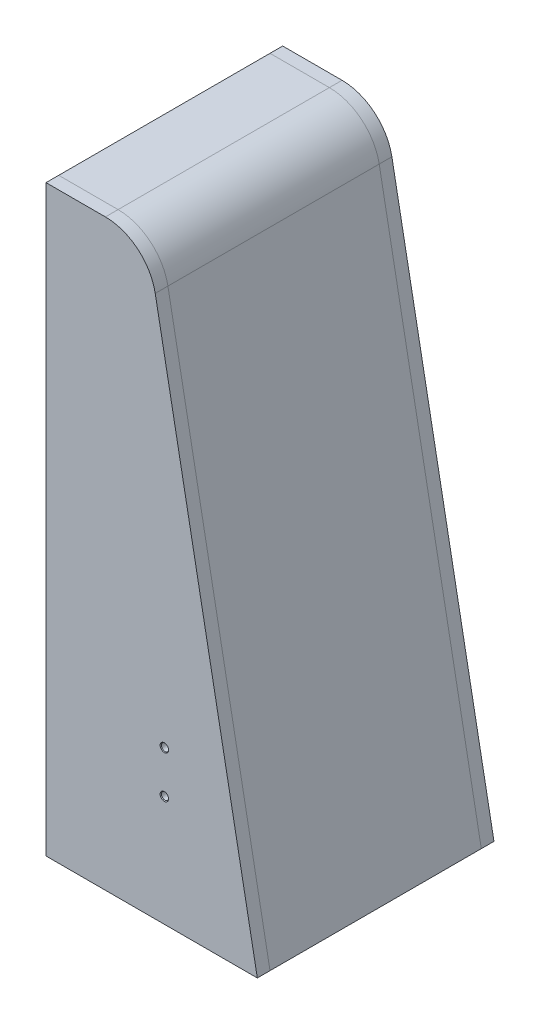
SolidWorks part; units mm, degrees
material "Q345"
ref_plane "前视基准面" through (0, 0, 0) normal (0, 0, 1) x (1, 0, 0)
ref_plane "上视基准面" through (0, 0, 0) normal (0, 1, 0) x (1, 0, 0)
ref_plane "右视基准面" through (0, 0, 0) normal (1, 0, 0) x (0, 0, -1)
sketch "草图1" plane through (0, 0, 0) normal (0, 0, 1) x (1, 0, 0)
  line L0 (0, 0) -> (0, 690)
  line L1 (0, 690) -> (70.2487, 690)
  line L2 (129.2114, 641.1089) -> (250, 0)
  line L3 (250, 0) -> (0, 0)
  arc A0 (129.2114, 641.1089) -> (70.2487, 690) centre (70.2487, 630) ccw
  point P7 (120, 690)
  dimension "D4" = 60
  dimension "D1" = 690
  dimension "D2" = 120
  dimension "D3" = 250
extrude "凸台-拉伸1" add sketch "草图1" along normal blind 15
sketch "草图2" plane through (0, 0, 0) normal (0, 0, -1) x (-1, 0, 0)
  line L0 (0, 675) -> (-70.2487, 675)
  line L1 (-114.4707, 638.3317) -> (-234.7361, 0)
  line L2 (0, 690) -> (0, 675)
  line L3 (-250, 0) -> (-234.7361, 0)
  line L4 (-250, 0) -> (0, 0)
  line L5 (0, 0) -> (0, 690)
  line L6 (0, 690) -> (-70.2487, 690)
  line L7 (-129.2114, 641.1089) -> (-250, 0)
  line L9 (-114.4707, 638.3317) -> (-235.2593, -2.7772) construction
  line L10 (0, 690) -> (-70.2487, 690)
  line L11 (-129.2114, 641.1089) -> (-250, 0)
  arc A0 (-70.2487, 675) -> (-114.4707, 638.3317) centre (-70.2487, 630) ccw
  arc A1 (-70.2487, 690) -> (-129.2114, 641.1089) centre (-70.2487, 630) ccw
  arc A2 (-70.2487, 690) -> (-129.2114, 641.1089) centre (-70.2487, 630) ccw
  dimension "D1" = 0
  dimension "D2" = 15
extrude "凸台-拉伸2" add sketch "草图2" along normal blind 250 separate body
sketch "草图3" plane through (0, 0, -250) normal (0, 0, -1) x (-1, 0, 0)
  line L4 (-250, 0) -> (0, 0)
  line L5 (-129.2114, 641.1089) -> (-250, 0)
  line L6 (0, 690) -> (-70.2487, 690)
  line L7 (0, 0) -> (0, 690)
  line L8 (-250, 0) -> (0, 0)
  line L9 (-129.2114, 641.1089) -> (-250, 0)
  line L10 (0, 690) -> (-70.2487, 690)
  line L11 (0, 0) -> (0, 690)
  arc A1 (-70.2487, 690) -> (-129.2114, 641.1089) centre (-70.2487, 630) ccw
  arc A2 (-70.2487, 690) -> (-129.2114, 641.1089) centre (-70.2487, 630) ccw
  dimension "D1" = 0
extrude "凸台-拉伸3" add sketch "草图3" along normal blind 15 separate body
sketch "草图4" plane through (0, 0, 15) normal (0, 0, 1) x (1, 0, 0)
  line L0 (140, 181) -> (140, 131) construction
  line L1 (0, 690) -> (0, 0) construction
  line L2 (0, 0) -> (250, 0) construction
  dimension "D1" = 50
  dimension "D2" = 140
  dimension "D3" = 131
hole_wizard "M10 螺纹孔1" positions "3D草图1" profile "草图5" tap size "M10" standard "GB" end condition up to next
sketch3d "3D草图1"
  point P0 (140, 181, 15)
  point P3 (140, 131, 15)
sketch "草图5" plane through (140, 181, 15) normal (1, 0, 0) x (0, -1, 0)
  line L0 (0, 0) -> (0, 15)
  line L1 (0, 15) -> (4.25, 15)
  line L2 (4.25, 15) -> (4.25, 0.775)
  line L3 (4.25, 0.775) -> (5.025, 0)
  line L5 (5.025, 0) -> (0, 0)
  line L6 (-4.25, 0.775) -> (-5.025, 0) construction
  line L11 (0, -6.35) -> (0, 107.95) construction
  dimension "通孔螺纹孔钻头直径" = 8.5
  dimension "通孔螺纹孔钻头深度" = 15
  dimension "近端锥形沉头孔直径" = 10.05
  dimension "近端锥形沉头孔角度" = 90
cosmetic thread "孔螺蚊线1" parameters "D2"=10
cosmetic thread "孔螺蚊线2" parameters "D2"=10
sketch "草图6" plane through (0, 0, -265) normal (0, 0, -1) x (-1, 0, 0)
  line L0 (0, 690) -> (-70.2487, 690) construction
  line L1 (-115, 590) -> (-45, 590)
  line L2 (-115, 590) -> (-115, 530)
  line L3 (-115, 530) -> (-45, 530)
  line L4 (-45, 590) -> (-45, 530)
  line L5 (-115, 590) -> (-45, 530) construction
  line L6 (-115, 530) -> (-45, 590) construction
  line L7 (0, 0) -> (0, 690) construction
  point P0 (-80, 560)
  dimension "D1" = 100
  dimension "D2" = 45
  dimension "D3" = 70
  dimension "D4" = 60
hole_wizard "M12 螺纹孔1" positions "3D草图3" profile "草图7" tap size "M12" standard "GB" end condition up to next
sketch3d "3D草图3"
  point P0 (45, 590, -265)
  point P3 (115, 590, -265)
  point P6 (115, 530, -265)
  point P9 (45, 530, -265)
sketch "草图7" plane through (45, 590, -265) normal (1, 0, 0) x (0, 1, 0)
  line L0 (0, 0) -> (0, 15.001)
  line L1 (0, 15.001) -> (5.1, 15.001)
  line L2 (5.1, 15.001) -> (5.1, 0.925)
  line L3 (5.1, 0.925) -> (6.025, 0)
  line L5 (6.025, 0) -> (0, 0)
  line L6 (-5.1, 0.925) -> (-6.025, 0) construction
  line L11 (0, -6.35) -> (0, 107.95) construction
  dimension "通孔螺纹孔钻头直径" = 10.2
  dimension "通孔螺纹孔钻头深度" = 15.001
  dimension "近端锥形沉头孔直径" = 12.05
  dimension "近端锥形沉头孔角度" = 90
cosmetic thread "孔螺蚊线3" parameters "D2"=12
cosmetic thread "孔螺蚊线4" parameters "D2"=12
cosmetic thread "孔螺蚊线5" parameters "D2"=12
cosmetic thread "孔螺蚊线6" parameters "D2"=12
